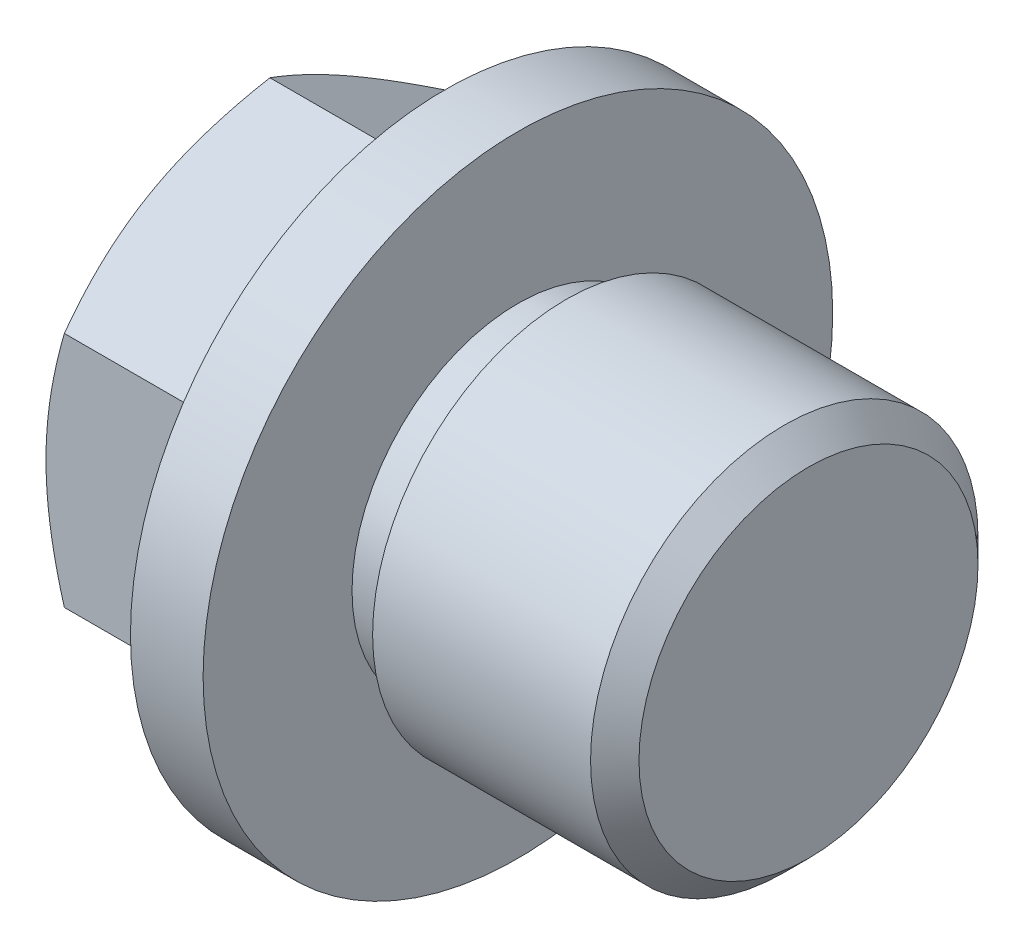
SolidWorks part; units mm, degrees
ref_plane "Front Plane" through (0, 0, 0) normal (0, 0, 1) x (1, 0, 0)
ref_plane "Top Plane" through (0, 0, 0) normal (0, 1, 0) x (1, 0, 0)
ref_plane "Right Plane" through (0, 0, 0) normal (1, 0, 0) x (0, 0, -1)
sketch "Sketch2" plane through (0, 0, 0) normal (1, 0, 0) x (0, 0, -1)
  line L1 (8.487, -4.9) -> (8.487, 4.9)
  line L2 (8.487, 4.9) -> (0, 9.8)
  line L3 (0, 9.8) -> (-8.487, 4.9)
  line L4 (-8.487, 4.9) -> (-8.487, -4.9)
  line L5 (-8.487, -4.9) -> (0, -9.8)
  line L6 (0, -9.8) -> (8.487, -4.9)
  circle A0 centre (0, 0) radius 8.487 construction
  dimension "D1" = 19.6
extrude "Boss-Extrude1" add sketch "Sketch2" along normal blind 8
sketch "Sketch3" plane through (0, 0, 0) normal (0, 1, 0) x (1, 0, 0)
  line L0 (0, -8.487) -> (0, -27.1669)
  line L1 (0, -27.1669) -> (10.7848, -27.1669)
  line L2 (10.7848, -27.1669) -> (0, -8.487)
  line L3 (0, 0) -> (0, -8.487) construction
  line L4 (0, 0) -> (19.1271, 0) construction
  dimension "D1" = 30
revolve "Cut-Revolve1" cut sketch "Sketch3" angle 360 about L4
sketch "Sketch4" plane through (0, 0, 0) normal (0, 0, 1) x (1, 0, 0)
  line L0 (8, 0) -> (8, 13)
  line L1 (8, 4.9) -> (8, -4.9) construction
  line L2 (8, 13) -> (11, 13)
  line L3 (11, 13) -> (11, 6.85)
  line L4 (11, 6.85) -> (13, 6.85)
  line L5 (13, 6.85) -> (13, 8)
  line L6 (13, 8) -> (23, 8)
  line L7 (23, 8) -> (23, 0)
  line L8 (23, 0) -> (8, 0)
  line L9 (-2.2123, 0) -> (23.9669, 0) construction
  dimension "D1" = 26
  dimension "D2" = 16
  dimension "D3" = 13.7
  dimension "D4" = 2
  dimension "D5" = 23
  dimension "D6" = 3
revolve "Revolve1" add sketch "Sketch4" angle 360 about L9
cosmetic thread "Cosmetic Thread1" parameters "D2"=13.6
chamfer "Chamfer1" distance 1 angle 45 1 edges at (23, 0, 8)
sketch "Sketch5" plane through (0, 0, 0) normal (-1, 0, 0) x (0, 0, 1)
  line L0 (-6.061, -1.4568) -> (6.4567, -1.0252) construction
  text T0 "放油螺栓" font "汉仪长仿宋体" height in points 6
extrude "Boss-Extrude2" add sketch "Sketch5" along normal blind 0.1
